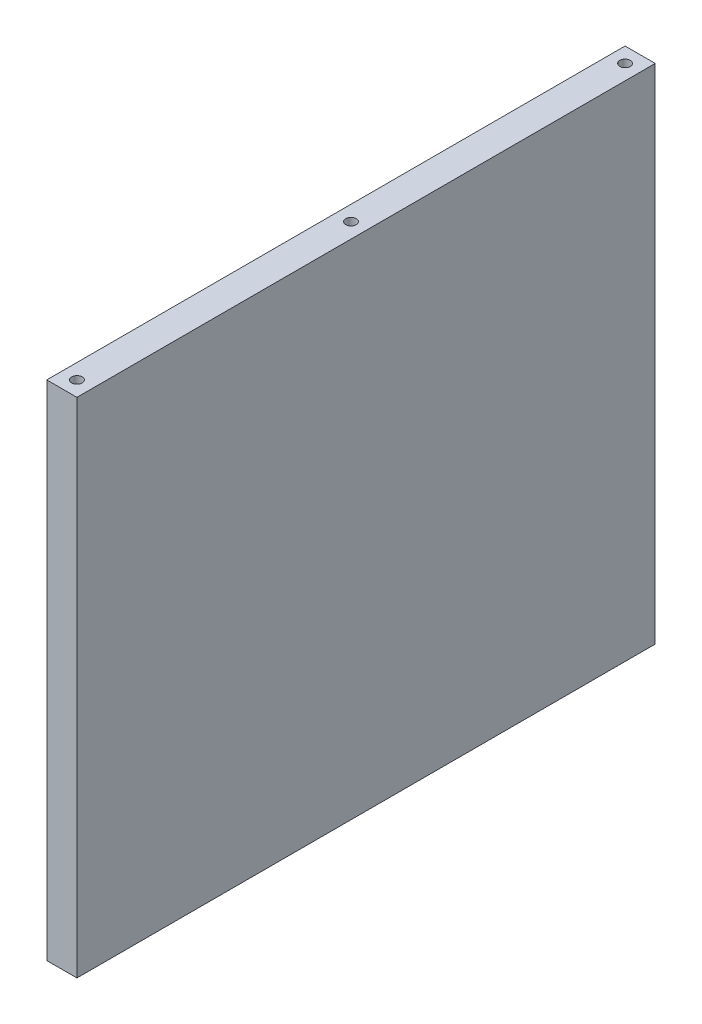
from build123d import *

# Parameters (mm, degrees)
SKETCH1_W                  = 230
SKETCH1_H                  = 200
BOSS_EXTRUDE1_DEPTH        = 6
M5_TAPPED_HOLE1_AT_2_COUNT = 2
M5_TAPPED_HOLE1_AT_2_PITCH = 109
M5_TAPPED_HOLE1_AT_3_COUNT = 2
M5_TAPPED_HOLE1_AT_3_PITCH = 218


with BuildPart() as part:
    # Sketch1 → Boss-Extrude1 (new, symmetric)
    with BuildSketch(Plane(origin=(0, 0, 0), x_dir=(0, 0, -1), z_dir=(1, 0, 0))):
        Rectangle(SKETCH1_W, SKETCH1_H)
    extrude(amount=BOSS_EXTRUDE1_DEPTH, both=True)

    # Sketch3 → M5 Tapped Hole1 (revolve, cut)
    with BuildSketch(Plane(origin=(0, 100, -109), x_dir=(0, 0, 1), z_dir=(1, 0, 0))):
        Polygon((0, 0), (0, 25.7618073), (2.1, 24.5), (2.1, 0), align=None)
    m5_tapped_hole1 = revolve(axis=Axis((0, 106.35, -109), (0, -1, 0)), mode=Mode.SUBTRACT)

    # M5 Tapped Hole1 at 2: M5 Tapped Hole1 ×2
    with Locations(*[(0, 0, i * M5_TAPPED_HOLE1_AT_2_PITCH) for i in range(1, M5_TAPPED_HOLE1_AT_2_COUNT)]):
        add(m5_tapped_hole1, mode=Mode.SUBTRACT)

    # M5 Tapped Hole1 at 3: M5 Tapped Hole1 ×2
    with Locations(*[(0, 0, i * M5_TAPPED_HOLE1_AT_3_PITCH) for i in range(1, M5_TAPPED_HOLE1_AT_3_COUNT)]):
        add(m5_tapped_hole1, mode=Mode.SUBTRACT)

    # Mirror1: M5 Tapped Hole1 across plane
    add(m5_tapped_hole1.mirror(Plane.ZX), mode=Mode.SUBTRACT)

    # Mirror1 copy 1 sketch → Mirror1 copy 1 (revolve, cut)
    with BuildSketch(Plane(origin=(0, -100, 0), x_dir=(0, 0, 1), z_dir=(1, 0, 0))):
        Polygon((0, 0), (0, -25.7618073), (2.1, -24.5), (2.1, 0), align=None)
    revolve(axis=Axis((0, -106.35, 0), (0, -1, 0)), mode=Mode.SUBTRACT)

    # Mirror1 copy 2 sketch → Mirror1 copy 2 (revolve, cut)
    with BuildSketch(Plane(origin=(0, -100, 109), x_dir=(0, 0, 1), z_dir=(1, 0, 0))):
        Polygon((0, 0), (0, -25.7618073), (2.1, -24.5), (2.1, 0), align=None)
    revolve(axis=Axis((0, -106.35, 109), (0, -1, 0)), mode=Mode.SUBTRACT)


solid = part.part
